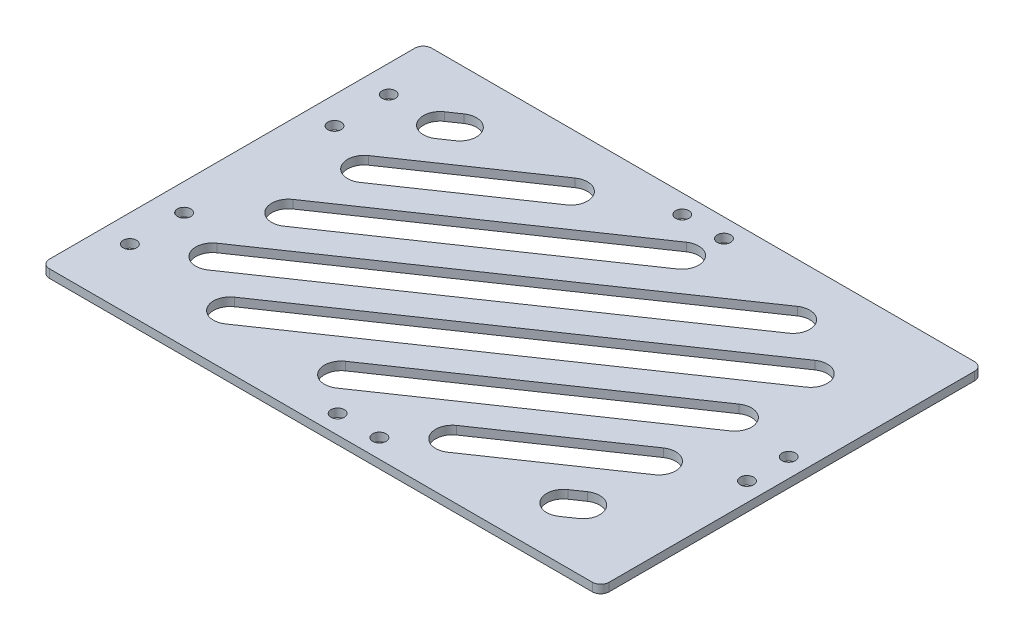
from build123d import *

# Parameters (mm, degrees)
SKETCH1_W               = 134
SKETCH1_H               = 91.5
SKETCH1_R               = 1.6
BOSS_EXTRUDE1_DEPTH     = 2
CUT_EXTRUDE2_DEPTH      = 82.982086458
CUT_EXTRUDE2_DEPTH_BACK = 82.982086458
R2_FILLET_1_R           = 2


with BuildPart() as part:
    # Sketch1 → Boss-Extrude1 (new body)
    with BuildSketch(Plane(origin=(0, 0, 0), x_dir=(1, 0, 0), z_dir=(0, 1, 0))):
        with Locations((1, 0)):
            Rectangle(SKETCH1_W, SKETCH1_H)
        with Locations(Location((-59.5, 31, 0), (0, 0, 270))):
            Circle(SKETCH1_R, mode=Mode.SUBTRACT)
        with Locations(Location((-59.5, 18, 0), (0, 0, 270))):
            Circle(SKETCH1_R, mode=Mode.SUBTRACT)
        with Locations(Location((-59.5, -18, 0), (0, 0, 90))):
            Circle(SKETCH1_R, mode=Mode.SUBTRACT)
        with Locations(Location((-59.5, -31, 0), (0, 0, 90))):
            Circle(SKETCH1_R, mode=Mode.SUBTRACT)
        with Locations(Location((63.5, 3.75, 0), (0, 0, 270))):
            Circle(SKETCH1_R, mode=Mode.SUBTRACT)
        with Locations(Location((63.5, -6.25, 0), (0, 0, 270))):
            Circle(SKETCH1_R, mode=Mode.SUBTRACT)
        with Locations(Location((0.5, -41.25, 0), (0, 0, 270))):
            Circle(SKETCH1_R, mode=Mode.SUBTRACT)
        with Locations(Location((10.5, -41.25, 0), (0, 0, 270))):
            Circle(SKETCH1_R, mode=Mode.SUBTRACT)
        with Locations(Location((10.5, 41.25, 0), (0, 0, 90))):
            Circle(SKETCH1_R, mode=Mode.SUBTRACT)
        with Locations(Location((0.5, 41.25, 0), (0, 0, 90))):
            Circle(SKETCH1_R, mode=Mode.SUBTRACT)
    extrude(amount=BOSS_EXTRUDE1_DEPTH)

    # Sketch5 → Cut-Extrude2 (cut, two sides: drawn at the far end of the back side and taken through both)
    with BuildSketch(Plane(origin=(0, 2, 0), x_dir=(1, 0, 0), z_dir=(0, 1, 0)).offset(-CUT_EXTRUDE2_DEPTH_BACK)):
        with BuildLine():
            Line((-49.255641565, 34.099169914), (-46.471955987, 35.999970141))
            ThreePointArc((-46.471955987, 35.999970141), (-40.91297049, 34.952267774), (-41.960672856, 29.393282278))
            Line((-41.960672856, 29.393282278), (-44.744358435, 27.492482051))
            ThreePointArc((-44.744358435, 27.492482051), (-50.303343931, 28.540184417), (-49.255641565, 34.099169914))
        make_face()
        with BuildLine():
            Line((-49.255641565, 15.935756946), (-19.871985084, 35.999970141))
            ThreePointArc((-19.871985084, 35.999970141), (-14.312999587, 34.952267774), (-15.360701954, 29.393282278))
            Line((-15.360701954, 29.393282278), (-44.744358435, 9.329069084))
            ThreePointArc((-44.744358435, 9.329069084), (-50.303343931, 10.37677145), (-49.255641565, 15.935756946))
        make_face()
        with BuildLine():
            Line((-49.255641565, -2.227656021), (6.727985819, 35.999970141))
            ThreePointArc((6.727985819, 35.999970141), (12.286971315, 34.952267774), (11.239268949, 29.393282278))
            Line((11.239268949, 29.393282278), (-44.744358435, -8.834343884))
            ThreePointArc((-44.744358435, -8.834343884), (-50.303343931, -7.786641517), (-49.255641565, -2.227656021))
        make_face()
        with BuildLine():
            Line((-49.255641565, -20.391068988), (33.327956722, 35.999970141))
            ThreePointArc((33.327956722, 35.999970141), (38.886942218, 34.952267774), (37.839239852, 29.393282278))
            Line((37.839239852, 29.393282278), (-44.744358435, -26.997756851))
            ThreePointArc((-44.744358435, -26.997756851), (-50.303343931, -25.950054485), (-49.255641565, -20.391068988))
        make_face()
        with BuildLine():
            Line((-35.955656114, -29.472775472), (46.627942173, 26.918263657))
            ThreePointArc((46.627942173, 26.918263657), (52.18692767, 25.870561291), (51.139225303, 20.311575794))
            Line((51.139225303, 20.311575794), (-31.444372983, -36.079463334))
            ThreePointArc((-31.444372983, -36.079463334), (-37.00335848, -35.031760968), (-35.955656114, -29.472775472))
        make_face()
        with BuildLine():
            Line((-9.355685211, -29.472775472), (46.627942173, 8.75485069))
            ThreePointArc((46.627942173, 8.75485069), (52.18692767, 7.707148324), (51.139225303, 2.148162827))
            Line((51.139225303, 2.148162827), (-4.844402081, -36.079463334))
            ThreePointArc((-4.844402081, -36.079463334), (-10.403387577, -35.031760968), (-9.355685211, -29.472775472))
        make_face()
        with BuildLine():
            Line((17.244285692, -29.472775472), (46.627942173, -9.408562277))
            ThreePointArc((46.627942173, -9.408562277), (52.18692767, -10.456264644), (51.139225303, -16.01525014))
            Line((51.139225303, -16.01525014), (21.755568822, -36.079463334))
            ThreePointArc((21.755568822, -36.079463334), (16.196583325, -35.031760968), (17.244285692, -29.472775472))
        make_face()
        with BuildLine():
            Line((43.844256595, -29.472775472), (46.627942173, -27.571975244))
            ThreePointArc((46.627942173, -27.571975244), (52.18692767, -28.619677611), (51.139225303, -34.178663107))
            Line((51.139225303, -34.178663107), (48.355539725, -36.079463334))
            ThreePointArc((48.355539725, -36.079463334), (42.796554228, -35.031760968), (43.844256595, -29.472775472))
        make_face()
    extrude(amount=CUT_EXTRUDE2_DEPTH + CUT_EXTRUDE2_DEPTH_BACK, mode=Mode.SUBTRACT)

    # R2 Fillet 1
    r2_fillet_1_edges = [part.edges().sort_by_distance(p)[0] for p in [
        (-66, 1, -45.75),
        (68, 1, -45.75),
        (68, 1, 45.75),
        (-66, 1, 45.75),
    ]]
    fillet(r2_fillet_1_edges, radius=R2_FILLET_1_R)


solid = part.part
